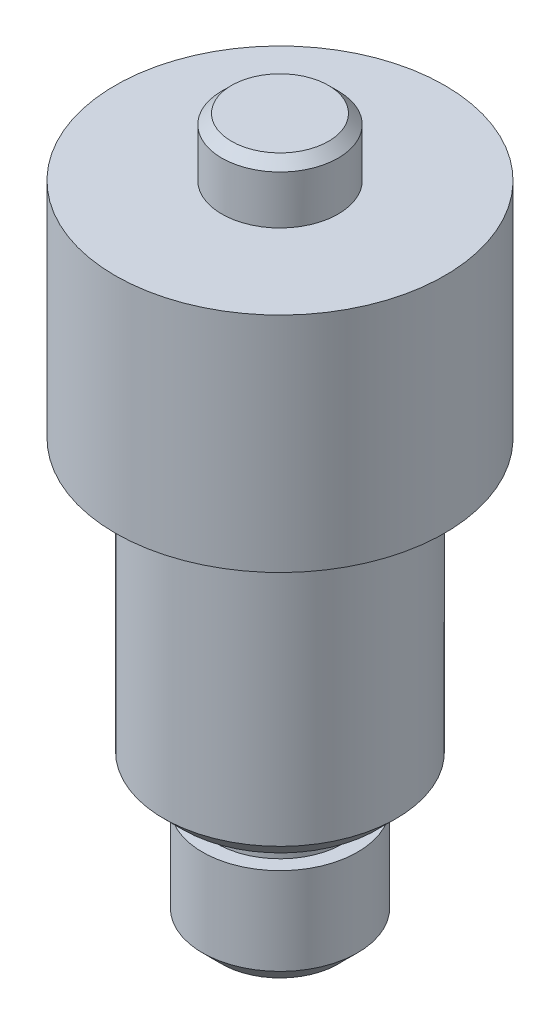
from build123d import *

# Parameters (mm, degrees)
CHAMFER_1_SIZE = 2
CHAMFER_2_SIZE = 1
FILLET_1_R     = 0.3


with BuildPart() as part:
    # 草图1 → 旋转1 (revolve)
    with BuildSketch(Plane.XY, mode=Mode.PRIVATE) as revolve_1_sk:
        Polygon((0, 0), (6, 0), (6, -6), (17, -6), (17, -29), (12, -29), (12, -59), (6.5, -59), (6.5, -62), (8, -62), (8, -73), (0, -73), align=None)
    revolve(revolve_1_sk.sketch.rotate(Axis((0, -73, 0), (0, 1, 0)), 90), axis=Axis((0, -73, 0), (0, 1, 0)))

    # 倒角1
    chamfer_1_edges = [part.edges().sort_by_distance(p)[0] for p in [
        (0, -59, 12),
        (0, -73, 8),
    ]]
    chamfer(chamfer_1_edges, length=CHAMFER_1_SIZE)

    # 倒角2
    chamfer_2_edges = [part.edges().sort_by_distance(p)[0] for p in [
        (0, 0, 6),
    ]]
    chamfer(chamfer_2_edges, length=CHAMFER_2_SIZE)

    # 圆角1
    fillet_1_edges = [part.edges().sort_by_distance(p)[0] for p in [
        (0, -29, 12),
    ]]
    fillet(fillet_1_edges, radius=FILLET_1_R)


solid = part.part
